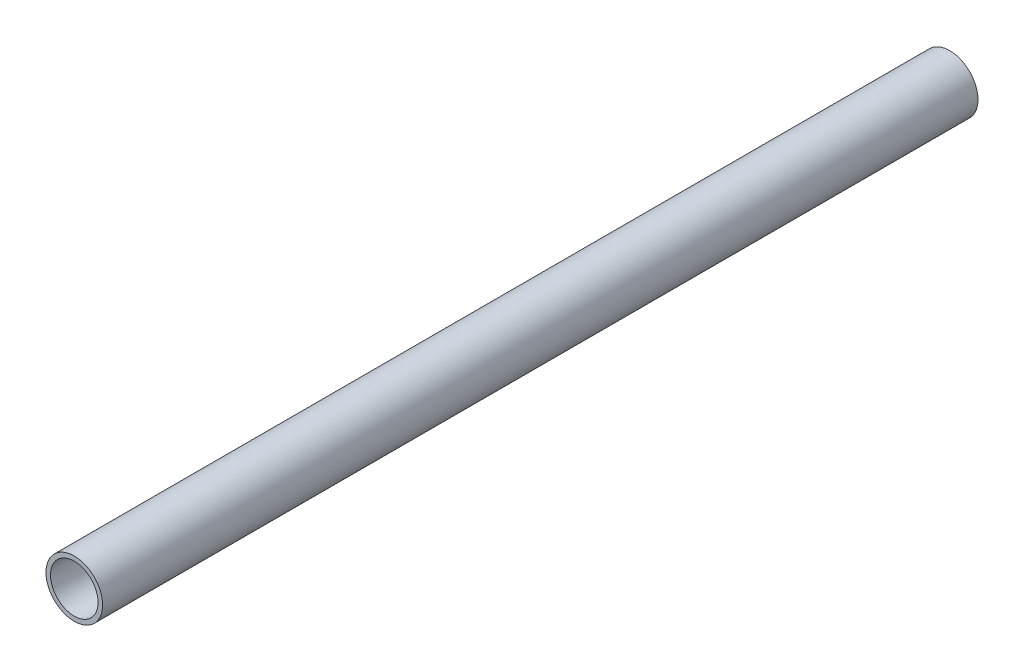
SolidWorks part; units mm, degrees
material "1023 碳钢板 (SS)"
ref_plane "前视基准面" through (0, 0, 0) normal (0, 0, 1) x (1, 0, 0)
ref_plane "上视基准面" through (0, 0, 0) normal (0, 1, 0) x (1, 0, 0)
ref_plane "右视基准面" through (0, 0, 0) normal (1, 0, 0) x (0, 0, -1)
sketch "草图1" plane through (0, 0, 0) normal (0, 0, 1) x (1, 0, 0)
  circle A0 centre (0, 0) radius 20
  dimension "D1" = 40
extrude "凸台-拉伸1" add sketch "草图1" along normal blind 618
shell "抽壳1" thickness 3.2
